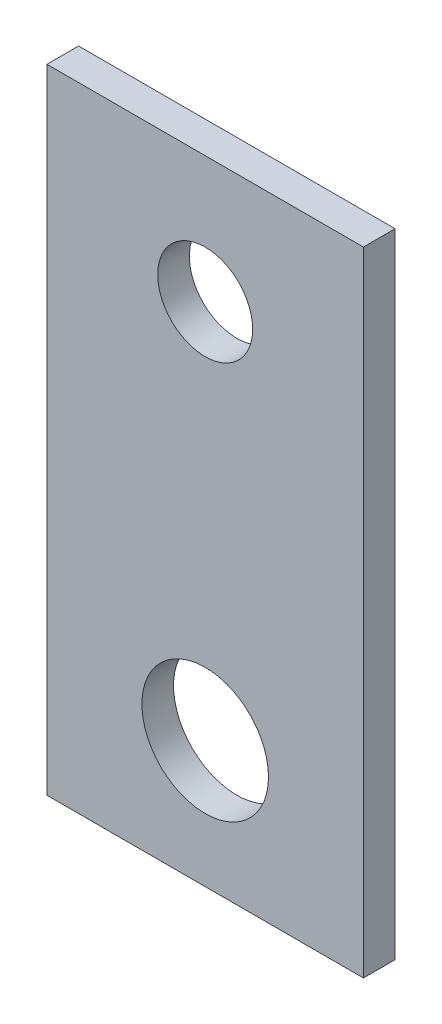
from build123d import *

# Parameters (mm, degrees)
SKETCH1_W           = 50
SKETCH1_H           = 100
BOSS_EXTRUDE1_DEPTH = 5
SKETCH2_R           = 10
SKETCH2_R_2         = 7.5
CUT_EXTRUDE1_DEPTH  = 5


with BuildPart() as part:
    # Sketch1 → Boss-Extrude1 (new body)
    with BuildSketch(Plane.XY):
        Rectangle(SKETCH1_W, SKETCH1_H)
    extrude(amount=BOSS_EXTRUDE1_DEPTH)

    # Sketch2 → Cut-Extrude1 (cut)
    with BuildSketch(Plane.XY.offset(5)):
        with Locations((0, -30)):
            Circle(SKETCH2_R)
        with Locations((0, 30)):
            Circle(SKETCH2_R_2)
    extrude(amount=-CUT_EXTRUDE1_DEPTH, mode=Mode.SUBTRACT)


solid = part.part
